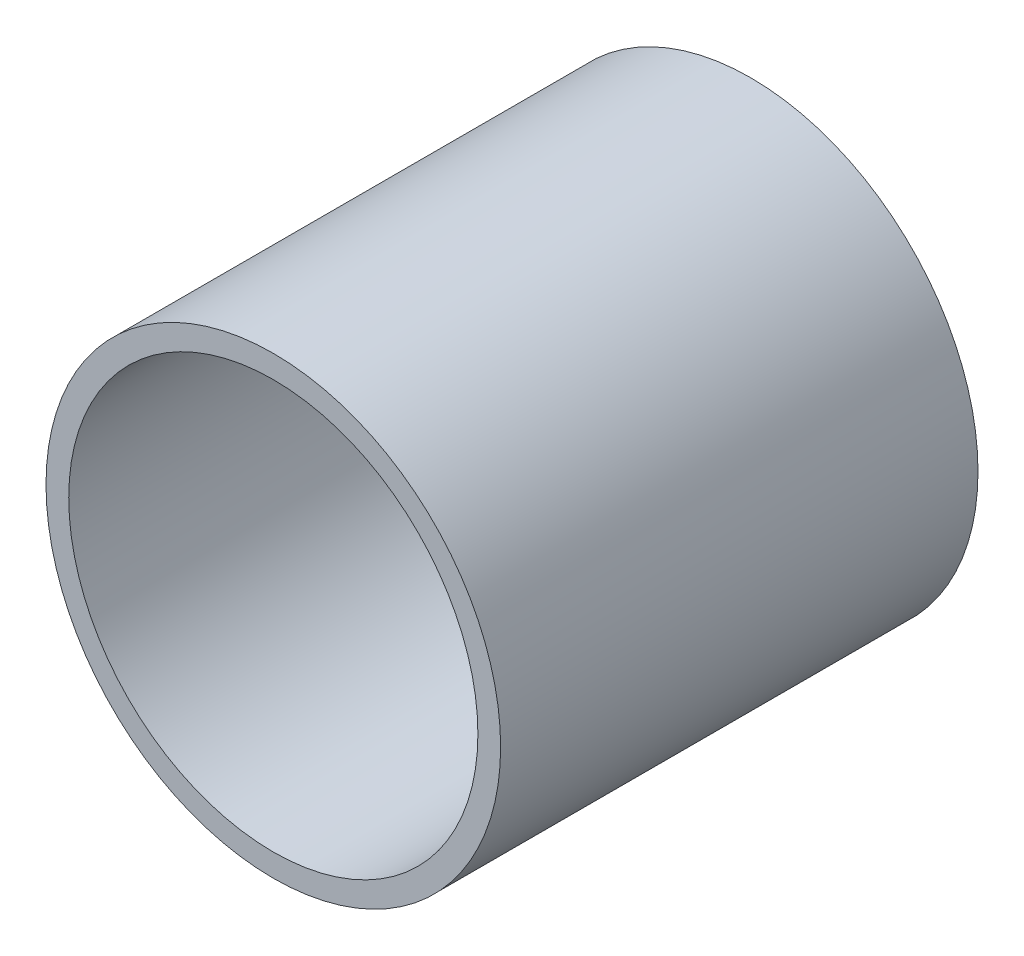
SolidWorks part; units mm, degrees
ref_plane "Front Plane" through (0, 0, 0) normal (0, 0, 1) x (1, 0, 0)
ref_plane "Top Plane" through (0, 0, 0) normal (0, 1, 0) x (1, 0, 0)
ref_plane "Right Plane" through (0, 0, 0) normal (1, 0, 0) x (0, 0, -1)
sketch "Sketch1" plane through (0, 0, 0) normal (0, 0, 1) x (1, 0, 0)
  circle A0 centre (0, 0) radius 9
  circle A1 centre (0, 0) radius 10
  dimension "D1" = 18
  dimension "D2" = 20
extrude "Boss-Extrude1" add sketch "Sketch1" along normal blind 21
